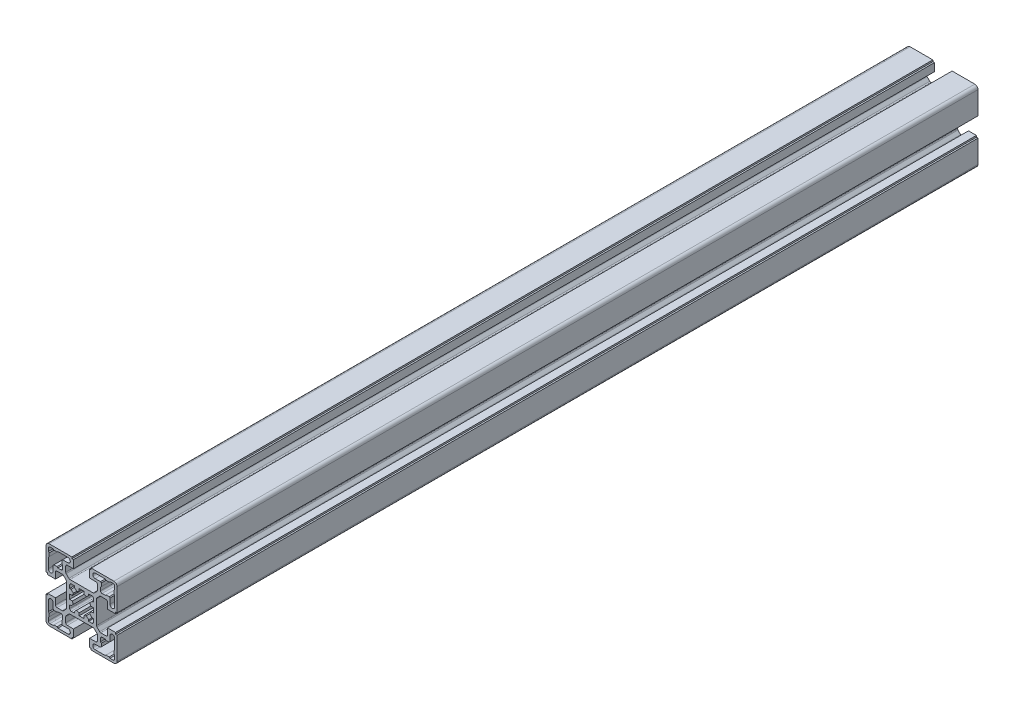
from build123d import *

# Parameters (mm, degrees)
EXTRUDE_1_DEPTH = 545


with BuildPart() as part:
    # 草图1 → 拉伸1 (new body)
    with BuildSketch(Plane.XY):
        with BuildLine():
            Line((33.706586033, 40.501982097), (35.388566549, 38.820001582))
            ThreePointArc((35.388566549, 38.820001582), (35.712989897, 38.603228831), (36.09567333, 38.527108363))
            Line((36.09567333, 38.527108363), (39.413692815, 38.527108363))
            ThreePointArc((39.413692815, 38.527108363), (40.120799596, 38.820001582), (40.413692815, 39.527108363))
            Line((40.413692815, 39.527108363), (40.413692815, 43.427108363))
            Line((40.413692815, 43.427108363), (45.413692815, 43.427108363))
            Line((45.413692815, 43.427108363), (45.413692815, 42.427108363))
            Line((45.413692815, 42.427108363), (46.413692815, 42.427108363))
            Line((46.413692815, 42.427108363), (46.413692815, 28.027108363))
            ThreePointArc((46.413692815, 28.027108363), (45.827906377, 26.612894801), (44.413692815, 26.027108363))
            Line((44.413692815, 26.027108363), (30.013692814, 26.027108363))
            Line((30.013692814, 26.027108363), (30.013692814, 27.027108363))
            Line((30.013692814, 27.027108363), (29.013692814, 27.027108363))
            Line((29.013692814, 27.027108363), (29.013692814, 32.027108363))
            Line((29.013692814, 32.027108363), (32.913692814, 32.027108363))
            ThreePointArc((32.913692814, 32.027108363), (33.620799596, 32.320001582), (33.913692814, 33.027108363))
            Line((33.913692814, 33.027108363), (33.913692814, 36.345127848))
            ThreePointArc((33.913692814, 36.345127848), (33.837572347, 36.72781128), (33.620799596, 37.052234629))
            Line((33.620799596, 37.052234629), (31.938819081, 38.734215144))
            ThreePointArc((31.938819081, 38.734215144), (31.614395732, 38.950987895), (31.231712299, 39.027108363))
            Line((31.231712299, 39.027108363), (16.59567333, 39.027108363))
            ThreePointArc((16.59567333, 39.027108363), (16.212989897, 38.950987895), (15.888566548, 38.734215144))
            Line((15.888566548, 38.734215144), (14.206586033, 37.052234629))
            ThreePointArc((14.206586033, 37.052234629), (13.989813282, 36.72781128), (13.913692814, 36.345127848))
            Line((13.913692814, 36.345127848), (13.913692814, 33.027108363))
            ThreePointArc((13.913692814, 33.027108363), (14.206586033, 32.320001582), (14.913692814, 32.027108363))
            Line((14.913692814, 32.027108363), (18.813692815, 32.027108363))
            Line((18.813692815, 32.027108363), (18.813692815, 27.027108363))
            Line((18.813692815, 27.027108363), (17.813692815, 27.027108363))
            Line((17.813692815, 27.027108363), (17.813692815, 26.027108363))
            Line((17.813692815, 26.027108363), (3.413692814, 26.027108363))
            ThreePointArc((3.413692814, 26.027108363), (1.999479252, 26.612894801), (1.413692814, 28.027108363))
            Line((1.413692814, 28.027108363), (1.413692814, 42.427108363))
            Line((1.413692814, 42.427108363), (2.413692814, 42.427108363))
            Line((2.413692814, 42.427108363), (2.413692814, 43.427108363))
            Line((2.413692814, 43.427108363), (7.413692814, 43.427108363))
            Line((7.413692814, 43.427108363), (7.413692814, 39.527108363))
            ThreePointArc((7.413692814, 39.527108363), (7.706586033, 38.820001582), (8.413692814, 38.527108363))
            Line((8.413692814, 38.527108363), (11.731712299, 38.527108363))
            ThreePointArc((11.731712299, 38.527108363), (12.114395732, 38.603228831), (12.43881908, 38.820001582))
            Line((12.43881908, 38.820001582), (14.120799595, 40.501982097))
            ThreePointArc((14.120799595, 40.501982097), (14.337572347, 40.826405446), (14.413692814, 41.209088878))
            Line((14.413692814, 41.209088878), (14.413692814, 55.845127848))
            ThreePointArc((14.413692814, 55.845127848), (14.337572347, 56.22781128), (14.120799595, 56.552234629))
            Line((14.120799595, 56.552234629), (12.43881908, 58.234215144))
            ThreePointArc((12.43881908, 58.234215144), (12.114395732, 58.450987896), (11.731712299, 58.527108363))
            Line((11.731712299, 58.527108363), (8.413692814, 58.527108363))
            ThreePointArc((8.413692814, 58.527108363), (7.706586033, 58.234215144), (7.413692814, 57.527108363))
            Line((7.413692814, 57.527108363), (7.413692814, 53.627108363))
            Line((7.413692814, 53.627108363), (2.413692814, 53.627108363))
            Line((2.413692814, 53.627108363), (2.413692814, 54.627108363))
            Line((2.413692814, 54.627108363), (1.413692814, 54.627108363))
            Line((1.413692814, 54.627108363), (1.413692814, 69.027108363))
            ThreePointArc((1.413692814, 69.027108363), (1.999479252, 70.441321926), (3.413692814, 71.027108363))
            Line((3.413692814, 71.027108363), (17.813692815, 71.027108363))
            Line((17.813692815, 71.027108363), (17.813692815, 70.027108363))
            Line((17.813692815, 70.027108363), (18.813692815, 70.027108363))
            Line((18.813692815, 70.027108363), (18.813692815, 65.027108363))
            Line((18.813692815, 65.027108363), (14.913692814, 65.027108363))
            ThreePointArc((14.913692814, 65.027108363), (14.206586033, 64.734215145), (13.913692814, 64.027108363))
            Line((13.913692814, 64.027108363), (13.913692814, 60.709088878))
            ThreePointArc((13.913692814, 60.709088878), (13.989813282, 60.326405446), (14.206586033, 60.001982097))
            Line((14.206586033, 60.001982097), (15.888566548, 58.320001582))
            ThreePointArc((15.888566548, 58.320001582), (16.212989897, 58.103228831), (16.59567333, 58.027108363))
            Line((16.59567333, 58.027108363), (31.231712299, 58.027108363))
            ThreePointArc((31.231712299, 58.027108363), (31.614395732, 58.103228831), (31.938819081, 58.320001582))
            Line((31.938819081, 58.320001582), (33.620799596, 60.001982097))
            ThreePointArc((33.620799596, 60.001982097), (33.837572347, 60.326405446), (33.913692814, 60.709088878))
            Line((33.913692814, 60.709088878), (33.913692814, 64.027108363))
            ThreePointArc((33.913692814, 64.027108363), (33.620799596, 64.734215145), (32.913692814, 65.027108363))
            Line((32.913692814, 65.027108363), (29.013692814, 65.027108363))
            Line((29.013692814, 65.027108363), (29.013692814, 70.027108363))
            Line((29.013692814, 70.027108363), (30.013692814, 70.027108363))
            Line((30.013692814, 70.027108363), (30.013692814, 71.027108363))
            Line((30.013692814, 71.027108363), (44.413692815, 71.027108363))
            ThreePointArc((44.413692815, 71.027108363), (45.827906377, 70.441321926), (46.413692815, 69.027108363))
            Line((46.413692815, 69.027108363), (46.413692815, 54.627108363))
            Line((46.413692815, 54.627108363), (45.413692815, 54.627108363))
            Line((45.413692815, 54.627108363), (45.413692815, 53.627108363))
            Line((45.413692815, 53.627108363), (40.413692815, 53.627108363))
            Line((40.413692815, 53.627108363), (40.413692815, 57.527108363))
            ThreePointArc((40.413692815, 57.527108363), (40.120799596, 58.234215144), (39.413692815, 58.527108363))
            Line((39.413692815, 58.527108363), (36.09567333, 58.527108363))
            ThreePointArc((36.09567333, 58.527108363), (35.712989897, 58.450987896), (35.388566549, 58.234215144))
            Line((35.388566549, 58.234215144), (33.706586033, 56.552234629))
            ThreePointArc((33.706586033, 56.552234629), (33.489813282, 56.22781128), (33.413692815, 55.845127848))
            Line((33.413692815, 55.845127848), (33.413692815, 41.209088878))
            ThreePointArc((33.413692815, 41.209088878), (33.489813282, 40.826405446), (33.706586033, 40.501982097))
        make_face()
        with BuildLine():
            Line((30.535013158, 44.027108363), (29.082272168, 45.479849354))
            ThreePointArc((29.082272168, 45.479849354), (29.45697001, 46.231007769), (29.723167834, 47.027108363))
            Line((29.723167834, 47.027108363), (31.413692814, 47.027108363))
            Line((31.413692814, 47.027108363), (31.413692814, 50.027108363))
            Line((31.413692814, 50.027108363), (29.723167834, 50.027108363))
            ThreePointArc((29.723167834, 50.027108363), (29.45697001, 50.823208957), (29.082272168, 51.574367373))
            Line((29.082272168, 51.574367373), (30.535013158, 53.027108363))
            Line((30.535013158, 53.027108363), (31.413692814, 53.027108363))
            Line((31.413692814, 53.027108363), (31.413692814, 55.027108363))
            ThreePointArc((31.413692814, 55.027108363), (31.120799596, 55.734215144), (30.413692814, 56.027108363))
            Line((30.413692814, 56.027108363), (28.413692814, 56.027108363))
            Line((28.413692814, 56.027108363), (28.413692814, 55.148428707))
            Line((28.413692814, 55.148428707), (26.960951824, 53.695687716))
            ThreePointArc((26.960951824, 53.695687716), (26.209793409, 54.070385558), (25.413692814, 54.336583382))
            Line((25.413692814, 54.336583382), (25.413692814, 56.027108363))
            Line((25.413692814, 56.027108363), (22.413692814, 56.027108363))
            Line((22.413692814, 56.027108363), (22.413692814, 54.336583382))
            ThreePointArc((22.413692814, 54.336583382), (21.61759222, 54.070385558), (20.866433805, 53.695687716))
            Line((20.866433805, 53.695687716), (19.413692814, 55.148428707))
            Line((19.413692814, 55.148428707), (19.413692814, 56.027108363))
            Line((19.413692814, 56.027108363), (17.413692814, 56.027108363))
            ThreePointArc((17.413692814, 56.027108363), (16.706586033, 55.734215144), (16.413692814, 55.027108363))
            Line((16.413692814, 55.027108363), (16.413692814, 53.027108363))
            Line((16.413692814, 53.027108363), (17.292372471, 53.027108363))
            Line((17.292372471, 53.027108363), (18.745113461, 51.574367373))
            ThreePointArc((18.745113461, 51.574367373), (18.370415619, 50.823208957), (18.104217795, 50.027108363))
            Line((18.104217795, 50.027108363), (16.413692814, 50.027108363))
            Line((16.413692814, 50.027108363), (16.413692814, 47.027108363))
            Line((16.413692814, 47.027108363), (18.104217795, 47.027108363))
            ThreePointArc((18.104217795, 47.027108363), (18.370415619, 46.231007769), (18.745113461, 45.479849354))
            Line((18.745113461, 45.479849354), (17.292372471, 44.027108363))
            Line((17.292372471, 44.027108363), (16.413692814, 44.027108363))
            Line((16.413692814, 44.027108363), (16.413692814, 42.027108363))
            ThreePointArc((16.413692814, 42.027108363), (16.706586033, 41.320001582), (17.413692814, 41.027108363))
            Line((17.413692814, 41.027108363), (19.413692814, 41.027108363))
            Line((19.413692814, 41.027108363), (19.413692814, 41.90578802))
            Line((19.413692814, 41.90578802), (20.866433805, 43.35852901))
            ThreePointArc((20.866433805, 43.35852901), (21.61759222, 42.983831168), (22.413692814, 42.717633344))
            Line((22.413692814, 42.717633344), (22.413692814, 41.027108363))
            Line((22.413692814, 41.027108363), (25.413692814, 41.027108363))
            Line((25.413692814, 41.027108363), (25.413692814, 42.717633344))
            ThreePointArc((25.413692814, 42.717633344), (26.209793409, 42.983831168), (26.960951824, 43.35852901))
            Line((26.960951824, 43.35852901), (28.413692814, 41.90578802))
            Line((28.413692814, 41.90578802), (28.413692814, 41.027108363))
            Line((28.413692814, 41.027108363), (30.413692814, 41.027108363))
            ThreePointArc((30.413692814, 41.027108363), (31.120799596, 41.320001582), (31.413692814, 42.027108363))
            Line((31.413692814, 42.027108363), (31.413692814, 44.027108363))
            Line((31.413692814, 44.027108363), (30.535013158, 44.027108363))
        make_face(mode=Mode.SUBTRACT)
        with BuildLine():
            Line((11.413692814, 66.027108363), (11.913692814, 66.527108364))
            Line((11.913692814, 66.527108364), (15.313692814, 66.527108364))
            ThreePointArc((15.313692814, 66.527108364), (16.813692814, 68.027108363), (15.313692814, 69.527108363))
            Line((15.313692814, 69.527108363), (8.913692815, 69.527108363))
            Line((8.913692815, 69.527108363), (8.413692814, 69.027108363))
            Line((8.413692814, 69.027108363), (6.413692814, 69.027108363))
            Line((6.413692814, 69.027108363), (5.913692814, 69.527108363))
            Line((5.913692814, 69.527108363), (3.913692814, 69.527108363))
            ThreePointArc((3.913692814, 69.527108363), (3.206586033, 69.234215145), (2.913692814, 68.527108363))
            Line((2.913692814, 68.527108363), (2.913692814, 66.527108363))
            Line((2.913692814, 66.527108363), (3.413692814, 66.027108363))
            Line((3.413692814, 66.027108363), (3.413692814, 64.027108363))
            Line((3.413692814, 64.027108363), (2.913692814, 63.527108363))
            Line((2.913692814, 63.527108363), (2.913692814, 57.127108364))
            ThreePointArc((2.913692814, 57.127108364), (4.413692814, 55.627108364), (5.913692814, 57.127108364))
            Line((5.913692814, 57.127108364), (5.913692814, 60.527108363))
            Line((5.913692814, 60.527108363), (6.413692814, 61.027108363))
            Line((6.413692814, 61.027108363), (8.413692814, 61.027108363))
            Line((8.413692814, 61.027108363), (8.913692814, 60.527108363))
            Line((8.913692814, 60.527108363), (10.913692814, 60.527108363))
            ThreePointArc((10.913692814, 60.527108363), (11.620799595, 60.820001582), (11.913692814, 61.527108363))
            Line((11.913692814, 61.527108363), (11.913692814, 63.527108363))
            Line((11.913692814, 63.527108363), (11.413692814, 64.027108363))
            Line((11.413692814, 64.027108363), (11.413692814, 66.027108363))
        make_face(mode=Mode.SUBTRACT)
        with BuildLine():
            Line((11.913692815, 30.527108363), (11.413692814, 31.027108363))
            Line((11.413692814, 31.027108363), (11.413692814, 33.027108363))
            Line((11.413692814, 33.027108363), (11.913692815, 33.527108363))
            Line((11.913692815, 33.527108363), (11.913692815, 35.527108363))
            ThreePointArc((11.913692815, 35.527108363), (11.620799596, 36.234215144), (10.913692815, 36.527108363))
            Line((10.913692815, 36.527108363), (8.913692815, 36.527108363))
            Line((8.913692815, 36.527108363), (8.413692815, 36.027108363))
            Line((8.413692815, 36.027108363), (6.413692814, 36.027108363))
            Line((6.413692814, 36.027108363), (5.913692814, 36.527108363))
            Line((5.913692814, 36.527108363), (5.913692814, 39.927108363))
            ThreePointArc((5.913692814, 39.927108363), (4.413692814, 41.427108363), (2.913692814, 39.927108363))
            Line((2.913692814, 39.927108363), (2.913692814, 33.527108363))
            Line((2.913692814, 33.527108363), (3.413692814, 33.027108363))
            Line((3.413692814, 33.027108363), (3.413692814, 31.027108363))
            Line((3.413692814, 31.027108363), (2.913692814, 30.527108363))
            Line((2.913692814, 30.527108363), (2.913692814, 28.527108363))
            ThreePointArc((2.913692814, 28.527108363), (3.206586033, 27.820001582), (3.913692814, 27.527108363))
            Line((3.913692814, 27.527108363), (5.913692814, 27.527108363))
            Line((5.913692814, 27.527108363), (6.413692814, 28.027108363))
            Line((6.413692814, 28.027108363), (8.413692814, 28.027108363))
            Line((8.413692814, 28.027108363), (8.913692815, 27.527108363))
            Line((8.913692815, 27.527108363), (15.313692814, 27.527108363))
            ThreePointArc((15.313692814, 27.527108363), (16.813692814, 29.027108363), (15.313692814, 30.527108363))
            Line((15.313692814, 30.527108363), (11.913692815, 30.527108363))
        make_face(mode=Mode.SUBTRACT)
        with BuildLine():
            Line((41.913692815, 36.527108363), (41.413692815, 36.027108363))
            Line((41.413692815, 36.027108363), (39.413692815, 36.027108363))
            Line((39.413692815, 36.027108363), (38.913692814, 36.527108363))
            Line((38.913692814, 36.527108363), (36.913692815, 36.527108363))
            ThreePointArc((36.913692815, 36.527108363), (36.206586033, 36.234215145), (35.913692815, 35.527108363))
            Line((35.913692815, 35.527108363), (35.913692815, 33.527108364))
            Line((35.913692815, 33.527108364), (36.413692815, 33.027108363))
            Line((36.413692815, 33.027108363), (36.413692815, 31.027108363))
            Line((36.413692815, 31.027108363), (35.913692815, 30.527108363))
            Line((35.913692815, 30.527108363), (32.513692815, 30.527108363))
            ThreePointArc((32.513692815, 30.527108363), (31.013692815, 29.027108363), (32.513692815, 27.527108363))
            Line((32.513692815, 27.527108363), (38.913692814, 27.527108363))
            Line((38.913692814, 27.527108363), (39.413692814, 28.027108363))
            Line((39.413692814, 28.027108363), (41.413692814, 28.027108363))
            Line((41.413692814, 28.027108363), (41.913692815, 27.527108363))
            Line((41.913692815, 27.527108363), (43.913692815, 27.527108363))
            ThreePointArc((43.913692815, 27.527108363), (44.620799596, 27.820001582), (44.913692815, 28.527108363))
            Line((44.913692815, 28.527108363), (44.913692815, 30.527108363))
            Line((44.913692815, 30.527108363), (44.413692814, 31.027108363))
            Line((44.413692814, 31.027108363), (44.413692814, 33.027108363))
            Line((44.413692814, 33.027108363), (44.913692815, 33.527108364))
            Line((44.913692815, 33.527108364), (44.913692815, 39.927108363))
            ThreePointArc((44.913692815, 39.927108363), (43.413692815, 41.427108363), (41.913692815, 39.927108363))
            Line((41.913692815, 39.927108363), (41.913692815, 36.527108363))
        make_face(mode=Mode.SUBTRACT)
        with BuildLine():
            Line((35.913692815, 66.527108363), (36.413692815, 66.027108363))
            Line((36.413692815, 66.027108363), (36.413692815, 64.027108363))
            Line((36.413692815, 64.027108363), (35.913692815, 63.527108363))
            Line((35.913692815, 63.527108363), (35.913692815, 61.527108363))
            ThreePointArc((35.913692815, 61.527108363), (36.206586033, 60.820001582), (36.913692815, 60.527108363))
            Line((36.913692815, 60.527108363), (38.913692814, 60.527108363))
            Line((38.913692814, 60.527108363), (39.413692815, 61.027108364))
            Line((39.413692815, 61.027108364), (41.413692815, 61.027108364))
            Line((41.413692815, 61.027108364), (41.913692815, 60.527108363))
            Line((41.913692815, 60.527108363), (41.913692815, 57.127108364))
            ThreePointArc((41.913692815, 57.127108364), (43.413692815, 55.627108364), (44.913692815, 57.127108364))
            Line((44.913692815, 57.127108364), (44.913692815, 63.527108363))
            Line((44.913692815, 63.527108363), (44.413692815, 64.027108363))
            Line((44.413692815, 64.027108363), (44.413692815, 66.027108363))
            Line((44.413692815, 66.027108363), (44.913692815, 66.527108363))
            Line((44.913692815, 66.527108363), (44.913692815, 68.527108363))
            ThreePointArc((44.913692815, 68.527108363), (44.620799596, 69.234215145), (43.913692815, 69.527108363))
            Line((43.913692815, 69.527108363), (41.913692815, 69.527108363))
            Line((41.913692815, 69.527108363), (41.413692814, 69.027108363))
            Line((41.413692814, 69.027108363), (39.413692814, 69.027108363))
            Line((39.413692814, 69.027108363), (38.913692814, 69.527108363))
            Line((38.913692814, 69.527108363), (32.513692815, 69.527108363))
            ThreePointArc((32.513692815, 69.527108363), (31.013692815, 68.027108363), (32.513692815, 66.527108363))
            Line((32.513692815, 66.527108363), (35.913692815, 66.527108363))
        make_face(mode=Mode.SUBTRACT)
    extrude(amount=EXTRUDE_1_DEPTH)


solid = part.part
